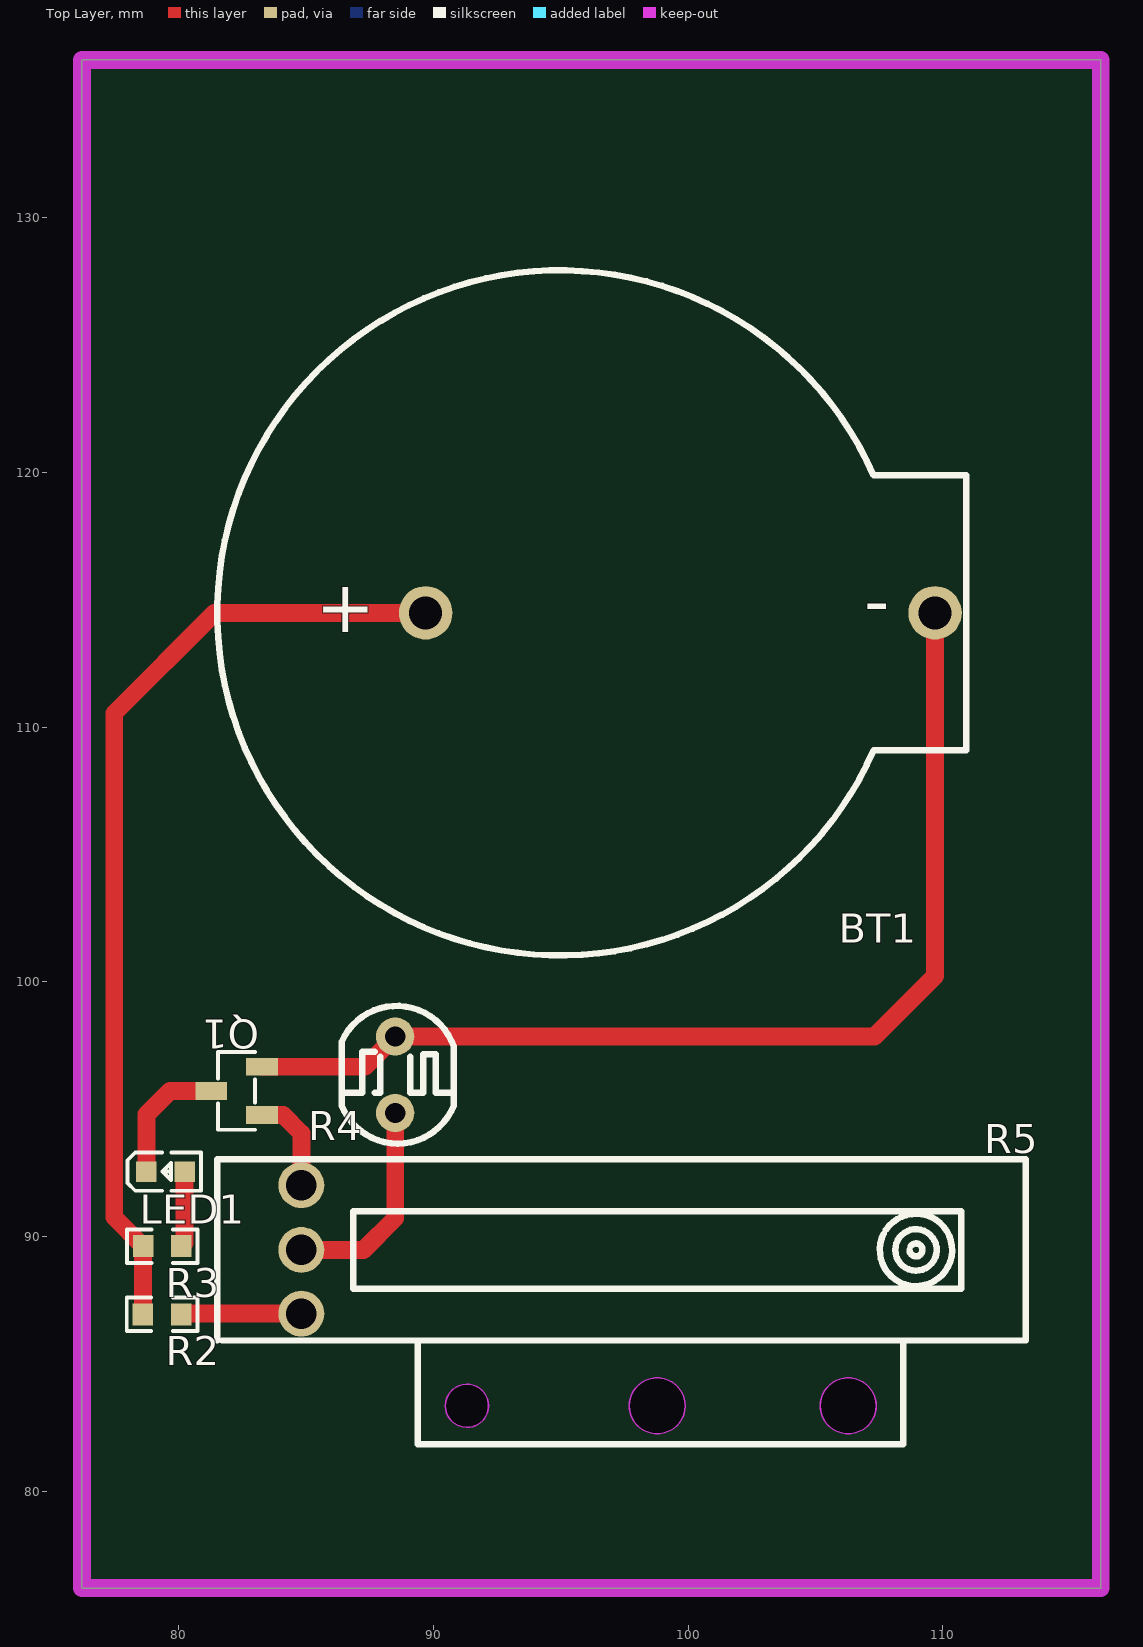
[diagram p0: Top Layer view]
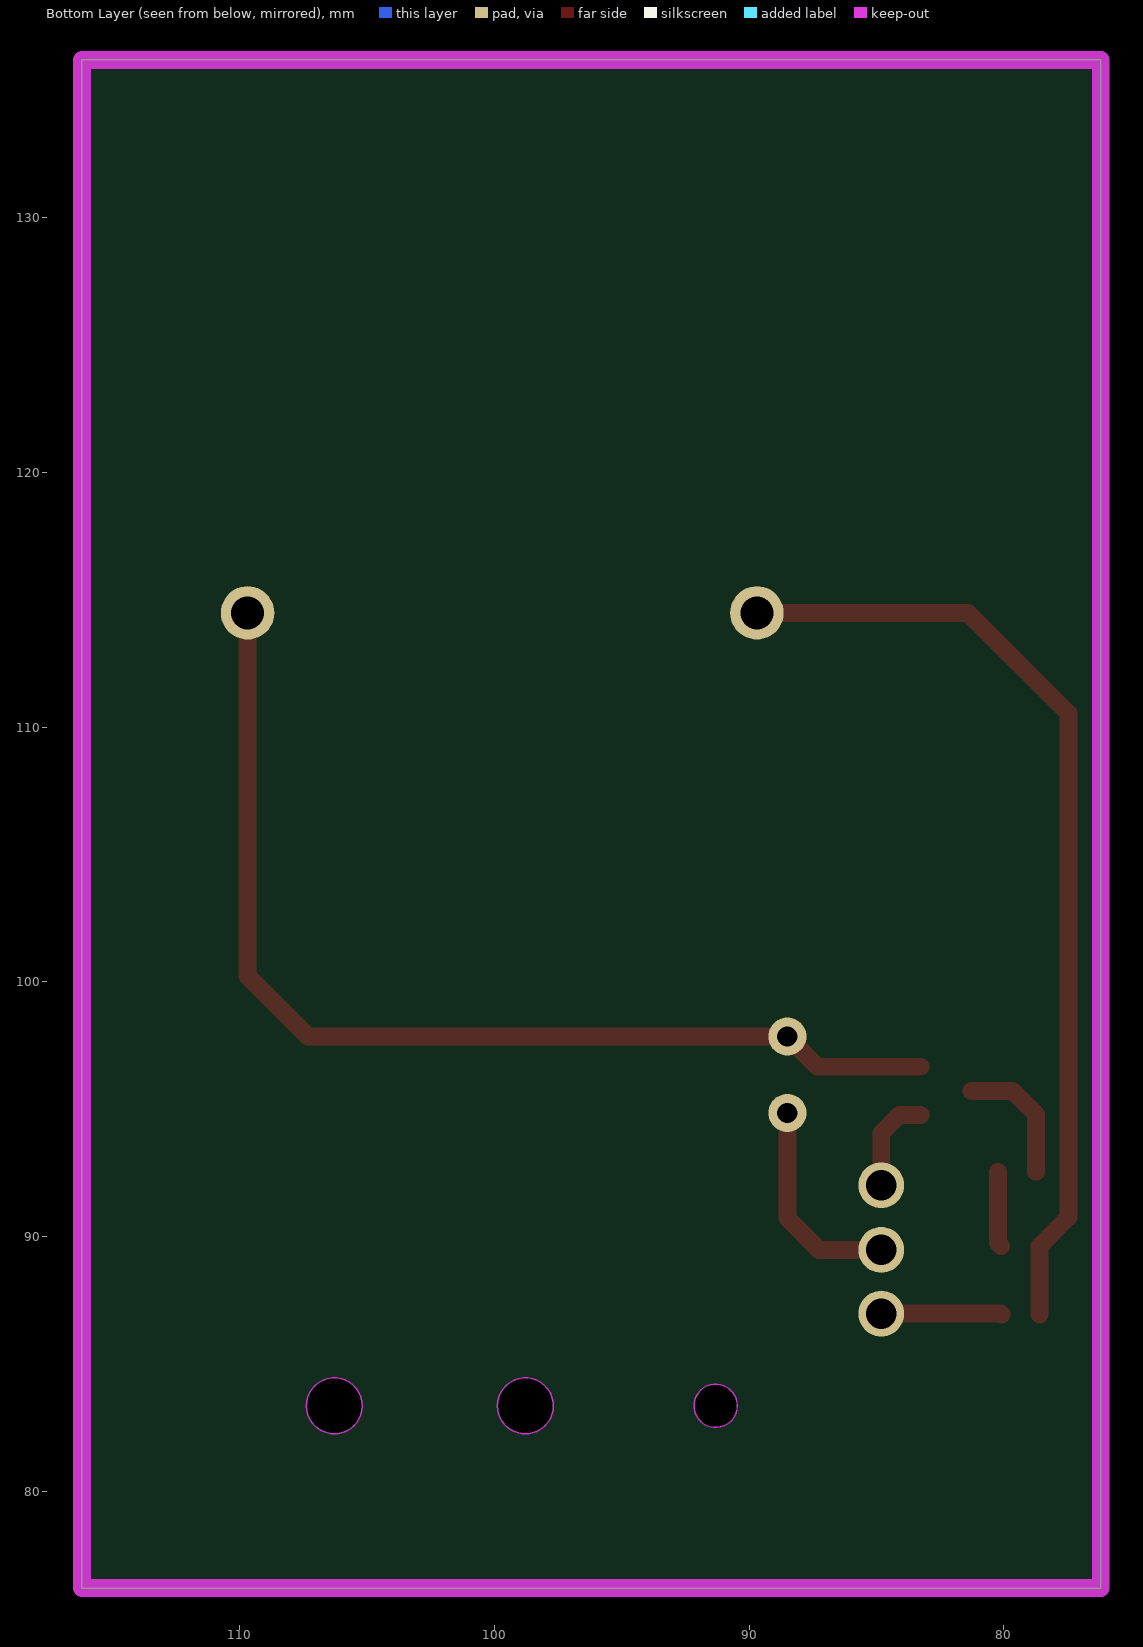
[diagram p1: Bottom Layer view, seen from below]
# Altium PCB MISC51971.pcbdoc
Units mm, origin at the board's own origin, x right, y up, seen from the top; angles counter-clockwise.
Board outline 40 x 60 mm, 2 copper layers (Top Layer, Bottom Layer), stack 1.58 mm thick; 7 components, 7 nets, 16 pads, 0 vias.

## Layer stack, top to bottom
Top Solder Mask Layer: solder mask 0.01, Dk 3.3
Top Layer: signal copper 0.035
Dielectric1: surface 1.51, FR4, Dk 4.5
Bottom Layer: signal copper 0.035
Bottom Solder Mask Layer: solder mask 0.01, Dk 3.3

## Board outline
76.2,136.2 76.2,76.2 116.2,76.2 116.2,136.2

## Design rules (kind name [scope] priority, off if disabled: settings)
BoardOutlineClearance copperThickness2oz_1 [All] p2 off: genericclearance=0.203 ignorepadtopadclearanceinfootprint=FALSE except(0: Arc-SplitContinuation Track-SplitContinuation SMDPad-SplitContinuation THPad-SplitContinuation Via-SplitContinuation Fill-SplitContinuation Region-SplitContinuation Poly-SplitContinuation Text-SplitContinuation Hole-SplitContinuation; 0.152: Arc-CutoutEdge SMDPad-CutoutEdge THPad-CutoutEdge Via-CutoutEdge Fill-CutoutEdge Region-CutoutEdge Text-CutoutEdge; 0.176: Hole-OutlineEdge Hole-CutoutEdge; 0.254: Poly-OutlineEdge Poly-CutoutEdge; 0.3: Arc-OutlineEdge Track-OutlineEdge SMDPad-OutlineEdge THPad-OutlineEdge Via-OutlineEdge Fill-OutlineEdge Region-OutlineEdge Text-OutlineEdge Track-CutoutEdge)
BoardOutlineClearance copperThickness1oz_1 [All] p4: genericclearance=0.102 ignorepadtopadclearanceinfootprint=FALSE except(0: Arc-SplitContinuation Track-SplitContinuation SMDPad-SplitContinuation THPad-SplitContinuation Via-SplitContinuation Fill-SplitContinuation Region-SplitContinuation Poly-SplitContinuation Text-SplitContinuation Hole-SplitContinuation; 0.152: SMDPad-CutoutEdge THPad-CutoutEdge Via-CutoutEdge Fill-CutoutEdge Region-CutoutEdge Text-CutoutEdge; 0.176: Hole-OutlineEdge Hole-CutoutEdge; 0.254: Poly-OutlineEdge Poly-CutoutEdge; 0.3: Arc-OutlineEdge Track-OutlineEdge SMDPad-OutlineEdge THPad-OutlineEdge Via-OutlineEdge Fill-OutlineEdge Region-OutlineEdge Text-OutlineEdge Arc-CutoutEdge Track-CutoutEdge)
Clearance copperThickness2oz [All] p1 off: gap=0.203 ignorepadtopadclearanceinfootprint=FALSE except(0.152: SMDPad-Track SMDPad-SMDPad THPad-Track SMDPad-THPad THPad-THPad Track-Via SMDPad-Via THPad-Via Via-Via Fill-Track Region-Track Fill-SMDPad Region-SMDPad Fill-THPad Region-THPad Fill-Via Region-Via Fill-Fill Fill-Region Region-Region Arc-Track Arc-SMDPad Arc-THPad Arc-Via Fill-Arc Region-Arc Arc-Arc Text-Track SMDPad-Text Text-THPad Text-Via Fill-Text Region-Text Arc-Text Text-Text; 0.176: Hole-Track Hole-SMDPad Hole-THPad Hole-Via Fill-Hole Region-Hole Hole-Arc Hole-Text; 0.254: Poly-Track Poly-SMDPad Poly-THPad Poly-Via Poly-Fill Poly-Region Poly-Poly Poly-Arc Poly-Text Poly-Hole)
Clearance copperThickness1oz [All] p3: gap=0.102 ignorepadtopadclearanceinfootprint=FALSE except(0.152: SMDPad-Track SMDPad-SMDPad THPad-Track SMDPad-THPad THPad-THPad Track-Via SMDPad-Via THPad-Via Via-Via Fill-Track Region-Track Fill-SMDPad Region-SMDPad Fill-THPad Region-THPad Fill-Via Region-Via Fill-Fill Fill-Region Region-Region Arc-Track Arc-SMDPad Arc-THPad Arc-Via Fill-Arc Region-Arc Arc-Arc Text-Track SMDPad-Text Text-THPad Text-Via Fill-Text Region-Text Arc-Text Text-Text; 0.176: Hole-Track Hole-SMDPad Hole-THPad Hole-Via Fill-Hole Region-Hole Hole-Arc Hole-Text; 0.254: Poly-Track Poly-SMDPad Poly-THPad Poly-Via Poly-Fill Poly-Region Poly-Poly Poly-Arc Poly-Text Poly-Hole)
DiffPairsRouting differentialPair [All] p1: maxlimit=0.152 minlimit=0.152 mostfreqgap=0.152 toplayer_minwidth=0.127 toplayer_prefwidth=0.254 toplayer_maxwidth=2.54 toplayer_mingap=0.152 toplayer_prefgap=0.152 toplayer_maxgap=0.152 bottomlayer_minwidth=0.127 bottomlayer_prefwidth=0.254 bottomlayer_maxwidth=2.54 bottomlayer_mingap=0.152 bottomlayer_prefgap=0.152 bottomlayer_maxgap=0.152 maxuncoupledlength=0.254
HoleToHoleClearance otherClearance [All] p1: gap=0.3 allowstackedmicrovias=TRUE
Length netLength [All] p1: minlimit=0 maxlimit=0
MatchedLengths netLengthTolerance [All] p1: tolerance=25.4
PasteMaskExpansion pasteMaskExpansion [All] p1: expansion=0
PlaneConnect innerPlane [All] p1: planeconnectstyle=Relief reliefexpansion=0.508 reliefentries=4 reliefconductorwidth=0.254 reliefairgap=0.254
PolygonConnect copperRegion [All] p1: connectstyle=Relief reliefconductorwidth=0.254 reliefentries=4 polygonreliefangle="90 Angle" airgapwidth=0.254 via.connectstyle=Relief via.reliefconductorwidth=0.254 via.reliefentries=4 via.polygonreliefangle="90 Angle" via.airgapwidth=0.254
RoutingVias viaSize [All] p1: holewidth=0.305 width=0.61 viastyle="Through Hole" minholewidth=0.3 minwidth=0.5 maxholewidth=6.3 maxwidth=10
SolderMaskExpansion solderMaskExpansion [IsVia] p1: expansion=-25.4 istentingtop=TRUE
SolderMaskExpansion solderMaskExpansion [All] p2: expansion=0.051 istentingtop=FALSE
Width copperThickness2oz_2 [All] p1 off: maxlimit=2.54 minlimit=0.203 preferedwidth=0.254
Width copperThickness1oz_2 [All] p2: maxlimit=2.54 minlimit=0.127 preferedwidth=0.254

## Components (designator, comment, footprint, x,y, rotation, side; value= is the part's Value field where it differs from the comment)
BT1 "79578211" BAT-TH_79578211 99.695,114.488 r180 top
LED1 "NCD0603Y2" LED0603-RD 79.483,92.546 r0 top
Q1 "SS8050" SOT-23-3_L2.9-W1.3-P1.90-LS2.4-BR 82.277,95.721 r0 top
R2 "10K" R0603 79.348,86.949 r180 top
R3 "10K" R0603 79.356,89.625 r180 top
R4 "GL5506(4-7K)" RES-TH_L5.1-W4.3-P3.00-D0.5 88.5,96.356 r90 top
R5 "10kΩ" RES-ADJ-TH_RDC1022A05 84.817,89.498 r180 top

## Footprints (in the part's own frame and the unit in brackets; to place one, negate y for a bottom-side part, rotate by r counter-clockwise, add the part's x,y. Pads: shape width x height; smd on the part's side, far side on the other; paste and mask are expansions set on the pad)
BAT-TH_79578211 [mm]
  round 2.1 hole 1.3: 1(-10,0) 2(10,0)
  silkscreen extent -11.22,-13.45 18.18,13.45
LED0603-RD [mm]
  rect 0.8x0.8 smd: 1(-0.749,0) 2(0.749,0)
  silkscreen extent -1.49,-0.75 1.39,0.76
R0603 [mm]
  rect 0.806x0.864 smd paste-100 mask+0.051: 1(-0.753,0) 2(0.753,0)
  silkscreen extent -1.39,-0.66 1.39,0.66
RES-ADJ-TH_RDC1022A05 [mm]
  round 1.8 hole 1.2: 1(0,0.02) 2(0,-2.52) 3(0,2.52)
  Board Outline Layer circle w0.003: c-21.47,6.14 r1.1
  Board Outline Layer circle w0.003: c-13.97,6.14 r1.1
  Board Outline Layer circle w0.003: c-6.5,6.14 r0.85
  Board Outline Layer region: -22.57,6.14 -22.461,6.617 -22.156,7 -21.715,7.212 -21.225,7.212 -20.784,7 -20.479,6.617 -20.37,6.14 -20.37,6.14 -20.479,5.663 -20.784,5.28 -21.225,5.068 -21.715,5.068 -22.156,5.28 -22.461,5.663 -22.57,6.14
  Board Outline Layer region: -22.57,6.14 -22.56,6.284 -22.532,6.425 -22.486,6.561 -22.422,6.69 -22.343,6.81 -22.248,6.918 -22.139,7.013 -22.02,7.093 -21.891,7.156 -21.755,7.202 -21.613,7.231 -21.47,7.24 -21.326,7.231 -21.185,7.202 -21.049,7.156 -20.92,7.093 -20.8,7.013 -20.692,6.918 -20.597,6.81 -20.517,6.69 -20.454,6.561 -20.407,6.425 -20.379,6.284 -20.37,6.14 -20.379,5.996 -20.407,5.855 -20.454,5.719 -20.517,5.59 -20.597,5.47 -20.692,5.362 -20.8,5.267 -20.92,5.187 -21.049,5.124 -21.185,5.077 -21.326,5.049 -21.47,5.04 -21.613,5.049 -21.755,5.077 -21.891,5.124 -22.02,5.187 -22.139,5.267 -22.248,5.362 -22.343,5.47 -22.422,5.59 -22.486,5.719 -22.532,5.855 -22.56,5.996
  Board Outline Layer region: -15.07,6.14 -14.961,6.617 -14.656,7 -14.215,7.212 -13.725,7.212 -13.284,7 -12.979,6.617 -12.87,6.14 -12.87,6.14 -12.979,5.663 -13.284,5.28 -13.725,5.068 -14.215,5.068 -14.656,5.28 -14.961,5.663 -15.07,6.14
  Board Outline Layer region: -15.07,6.14 -15.061,6.284 -15.033,6.425 -14.986,6.561 -14.923,6.69 -14.843,6.81 -14.748,6.918 -14.64,7.013 -14.52,7.093 -14.391,7.156 -14.255,7.202 -14.114,7.231 -13.97,7.24 -13.826,7.231 -13.685,7.202 -13.549,7.156 -13.42,7.093 -13.3,7.013 -13.192,6.918 -13.097,6.81 -13.017,6.69 -12.954,6.561 -12.907,6.425 -12.879,6.284 -12.87,6.14 -12.879,5.996 -12.907,5.855 -12.954,5.719 -13.017,5.59 -13.097,5.47 -13.192,5.362 -13.3,5.267 -13.42,5.187 -13.549,5.124 -13.685,5.077 -13.826,5.049 -13.97,5.04 -14.114,5.049 -14.255,5.077 -14.391,5.124 -14.52,5.187 -14.64,5.267 -14.748,5.362 -14.843,5.47 -14.923,5.59 -14.986,5.719 -15.033,5.855 -15.061,5.996
  Board Outline Layer region: -7.35,6.14 -7.266,6.509 -7.03,6.805 -6.689,6.969 -6.311,6.969 -5.97,6.805 -5.734,6.509 -5.65,6.14 -5.65,6.14 -5.734,5.771 -5.97,5.475 -6.311,5.311 -6.689,5.311 -7.03,5.475 -7.266,5.771 -7.35,6.14
  Board Outline Layer region: -7.35,6.14 -7.34,6.267 -7.312,6.39 -7.266,6.509 -7.202,6.619 -7.123,6.718 -7.03,6.805 -6.925,6.876 -6.81,6.931 -6.689,6.969 -6.563,6.988 -6.436,6.988 -6.311,6.969 -6.189,6.931 -6.075,6.876 -5.97,6.805 -5.877,6.718 -5.798,6.619 -5.734,6.509 -5.688,6.39 -5.659,6.267 -5.65,6.14 -5.659,6.013 -5.688,5.889 -5.734,5.771 -5.798,5.661 -5.877,5.562 -5.97,5.475 -6.075,5.404 -6.189,5.349 -6.311,5.311 -6.436,5.292 -6.563,5.292 -6.689,5.311 -6.81,5.349 -6.925,5.404 -7.03,5.475 -7.123,5.562 -7.202,5.661 -7.266,5.771 -7.312,5.889 -7.34,6.013
  Multi-Layer board cut-out: -22.57,6.14 -22.461,6.617 -22.156,7 -21.715,7.212 -21.225,7.212 -20.784,7 -20.479,6.617 -20.37,6.14 -20.37,6.14 -20.479,5.663 -20.784,5.28 -21.225,5.068 -21.715,5.068 -22.156,5.28 -22.461,5.663 -22.57,6.14
  Multi-Layer board cut-out: -15.07,6.14 -14.961,6.617 -14.656,7 -14.215,7.212 -13.725,7.212 -13.284,7 -12.979,6.617 -12.87,6.14 -12.87,6.14 -12.979,5.663 -13.284,5.28 -13.725,5.068 -14.215,5.068 -14.656,5.28 -14.961,5.663 -15.07,6.14
  Multi-Layer board cut-out: -7.35,6.14 -7.266,6.509 -7.03,6.805 -6.689,6.969 -6.311,6.969 -5.97,6.805 -5.734,6.509 -5.65,6.14 -5.65,6.14 -5.734,5.771 -5.97,5.475 -6.311,5.311 -6.689,5.311 -7.03,5.475 -7.266,5.771 -7.35,6.14
  silkscreen extent -28.45,-3.54 3.3,7.64
RES-TH_L5.1-W4.3-P3.00-D0.5 [mm]
  round 1.5 hole 0.8: 1(-1.5,0) 2(1.5,0)
  silkscreen extent -2.7,-2.3 2.7,2.1
SOT-23-3_L2.9-W1.3-P1.90-LS2.4-BR [mm]
  rect 1.25x0.7 smd: 1(1,-0.95) 2(1,0.95) 3(-1,0)
  silkscreen extent -0.73,-1.53 0.73,1.53

## Nets (pads, with @x,y where several pads share a name; then routed paths per layer and width w, separated by ;. In a path a pad name is that pad's centre, name@x,y a point inside that pad or via, vN(x,y) a via of type N, cw(c..) or ccw(c..) an arc to the next point about the centre after c; other vN are vias at no path point)
$1N2: LED1.1 Q1.3 | length 5.2
  Top Layer w0.7: LED1.1 78.734,94.797 79.658,95.721 Q1.3
$1N3: LED1.2 R3.1 | length 3
  Top Layer w0.7: R3.1 80.232,89.748 LED1.2
$1N4: R2.1 R5.3 | length 4.7
  Top Layer w0.7: R2.1 80.13,86.978 R5.3
$1N6: BT1.2 R2.2 R3.2 | length 37.9
  Top Layer w0.7: R2.2 78.603,86.958 R3.2 77.47,90.758 77.47,110.551 81.407,114.488 BT1.2
$1N7: BT1.1 Q1.2 R4.2 | length 42.1
  Top Layer w0.7: Q1.2 87.315,96.671 R4.2 107.32,97.856 109.695,100.231 BT1.1
$1N10: Q1.1 R5.2 | length 3.9
  Top Layer w0.7: Q1.1 84.106,94.771 84.817,94.06 R5.2
$1N11: R4.1 R5.1 | length 8.3
  Top Layer w0.7: R5.1 87.258,89.478 88.5,90.72 R4.1

## Keep-outs
Board Outline Layer:
  the board outline again, w0.7